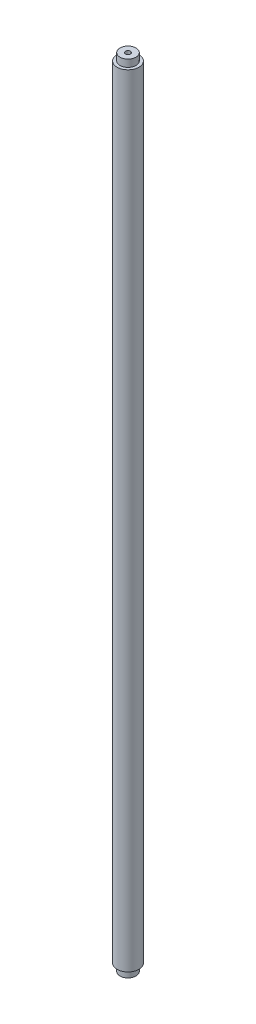
from build123d import *

# Parameters (mm, degrees)
SKETCH1_R             = 15
BOSS_EXTRUDE1_DEPTH   = 1075
SKETCH2_R             = 11
BOSS_EXTRUDE2_DEPTH   = 10
BOSS_EXTRUDE3_START   = 10
SKETCH3_R             = 11
BOSS_EXTRUDE3_DEPTH   = 10
M8_TAPPED_HOLE1_D     = 6.8
M8_TAPPED_HOLE1_DEPTH = 19.75
M8_TAPPED_HOLE1_TIP   = 2.042926105
M8_TAPPED_HOLE2_D     = 6.8
M8_TAPPED_HOLE2_DEPTH = 19.75
M8_TAPPED_HOLE2_TIP   = 2.042926105


with BuildPart() as part:
    # Sketch1 → Boss-Extrude1 (new body)
    with BuildSketch(Plane(origin=(0, 0, 0), x_dir=(1, 0, 0), z_dir=(0, 1, 0))):
        with Locations(Location((0, 0, 0), (0, 0, 270))):
            Circle(SKETCH1_R)
    extrude(amount=BOSS_EXTRUDE1_DEPTH)

    # Sketch2 → Boss-Extrude2 (add)
    with BuildSketch(Plane(origin=(0, 1075, 0), x_dir=(1, 0, 0), z_dir=(0, 1, 0))):
        with Locations(Location((0, 0, 0), (0, 0, 270))):
            Circle(SKETCH2_R)
    extrude(amount=BOSS_EXTRUDE2_DEPTH)

    # Sketch3 → Boss-Extrude3 (add)
    with BuildSketch(Plane.XZ.offset(BOSS_EXTRUDE3_START)):
        with Locations(Location((0, 0, 0), (0, 0, 90))):
            Circle(SKETCH3_R)
    extrude(amount=-BOSS_EXTRUDE3_DEPTH)

    # M8 Tapped Hole1
    with Locations(Plane(origin=(0, -10, 0), x_dir=(-1, 0, 0), z_dir=(0, -1, 0))):
        with Locations((0, 0)):
            Hole(M8_TAPPED_HOLE1_D / 2, depth=M8_TAPPED_HOLE1_DEPTH)
            with Locations((0, 0, -(M8_TAPPED_HOLE1_DEPTH + M8_TAPPED_HOLE1_TIP / 2))):  # 118° drill point
                Cone(0, M8_TAPPED_HOLE1_D / 2, M8_TAPPED_HOLE1_TIP, mode=Mode.SUBTRACT)

    # M8 Tapped Hole2
    with Locations(Plane(origin=(0, 1085, 0), x_dir=(1, 0, 0), z_dir=(0, 1, 0))):
        with Locations((0, 0)):
            Hole(M8_TAPPED_HOLE2_D / 2, depth=M8_TAPPED_HOLE2_DEPTH)
            with Locations((0, 0, -(M8_TAPPED_HOLE2_DEPTH + M8_TAPPED_HOLE2_TIP / 2))):  # 118° drill point
                Cone(0, M8_TAPPED_HOLE2_D / 2, M8_TAPPED_HOLE2_TIP, mode=Mode.SUBTRACT)


solid = part.part
